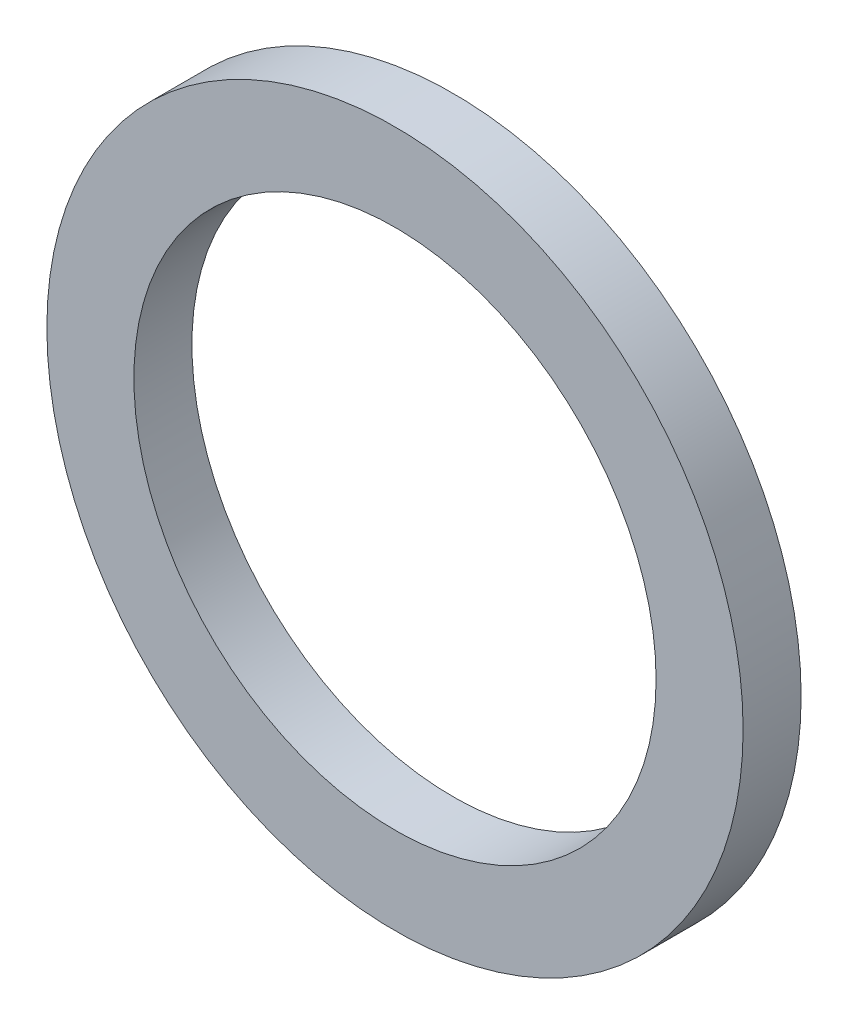
SolidWorks part; units mm, degrees
material "Q235B"
ref_plane "Front Plane" through (0, 0, 0) normal (0, 0, 1) x (1, 0, 0)
ref_plane "Top Plane" through (0, 0, 0) normal (0, 1, 0) x (1, 0, 0)
ref_plane "Right Plane" through (0, 0, 0) normal (1, 0, 0) x (0, 0, -1)
sketch "Sketch1" plane through (0, 0, 0) normal (0, 0, 1) x (1, 0, 0)
  circle A0 centre (0, 0) radius 30
  circle A1 centre (0, 0) radius 22.5
  dimension "D1" = 60
  dimension "D2" = 45
extrude "Boss-Extrude1" add sketch "Sketch1" along normal blind 5
